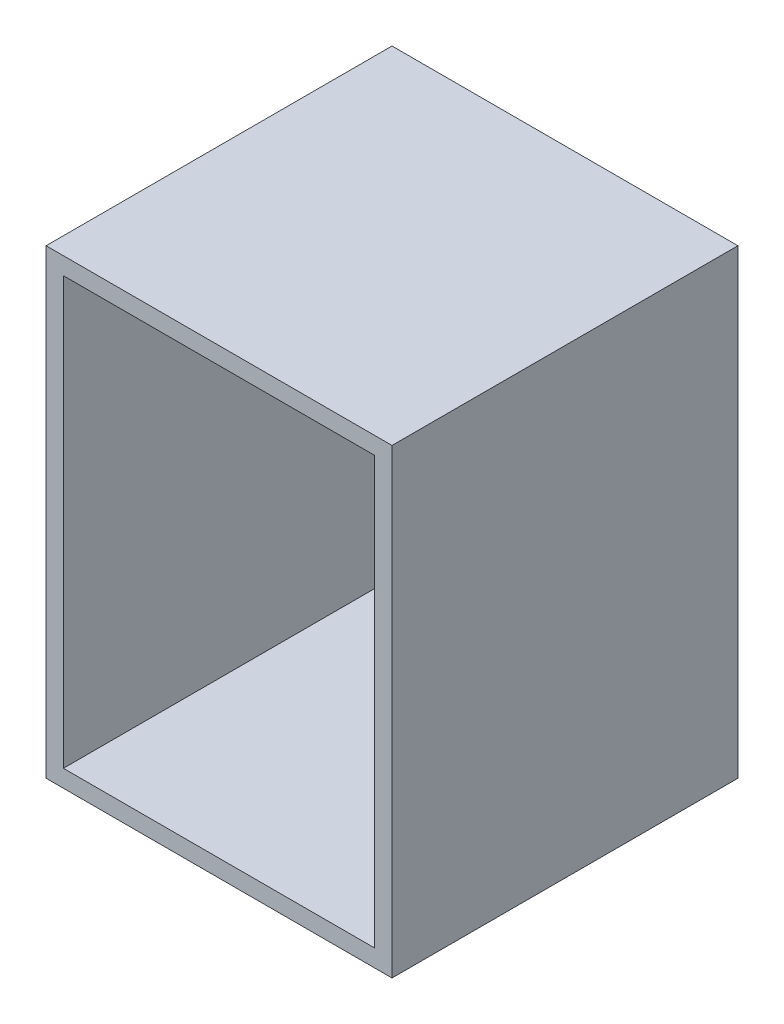
SolidWorks part; units mm, degrees
ref_plane "Front Plane" through (0, 0, 0) normal (0, 0, 1) x (1, 0, 0)
ref_plane "Top Plane" through (0, 0, 0) normal (0, 1, 0) x (1, 0, 0)
ref_plane "Right Plane" through (0, 0, 0) normal (1, 0, 0) x (0, 0, -1)
other "Configuration Table"
sketch "Sketch1" plane through (0, 0, 0) normal (0, 0, 1) x (1, 0, 0)
  line L0 (-37.0591, 39.2476) -> (-7.0591, 39.2476)
  line L1 (-7.0591, 39.2476) -> (-7.0591, -0.7524)
  line L2 (-7.0591, -0.7524) -> (-37.0591, -0.7524)
  line L3 (-37.0591, -0.7524) -> (-37.0591, 39.2476)
extrude "Boss-Extrude1" add sketch "Sketch1" along normal blind 30
sketch "Sketch2" plane through (0, 0, 30) normal (0, 0, 1) x (1, 0, 0)
  line L0 (-35.5591, 37.7476) -> (-8.5591, 37.7476)
  line L1 (-8.5591, 37.7476) -> (-8.5591, 0.7476)
  line L2 (-8.5591, 0.7476) -> (-35.5591, 0.7476)
  line L3 (-35.5591, 0.7476) -> (-35.5591, 37.7476)
  line L4 (-7.0591, -0.7524) -> (-7.0591, 39.2476) construction
  line L5 (-7.0591, 39.2476) -> (-37.0591, 39.2476) construction
  line L6 (-37.0591, -0.7524) -> (-7.0591, -0.7524) construction
  line L7 (-37.0591, 39.2476) -> (-37.0591, -0.7524) construction
  dimension "D1" = 1.5
  dimension "D2" = 1.5
  dimension "D3" = 1.5
  dimension "D4" = 1.5
extrude "Cut-Extrude1" cut sketch "Sketch2" against normal through all
